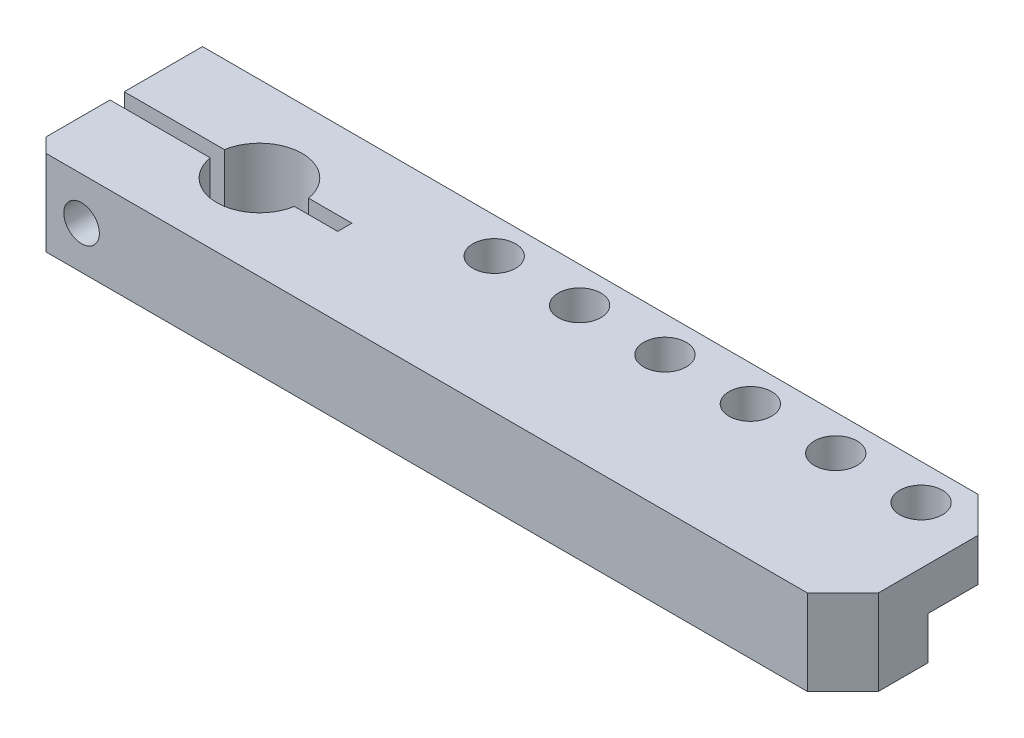
from build123d import *

# Parameters (mm, degrees)
SKETCH1_W                = 65
SKETCH1_H                = 12
SKETCH1_R                = 3
BOSS_EXTRUDE1_DEPTH      = 6
SKETCH2_W                = 32
SKETCH2_H                = 1
CUT_EXTRUDE1_DEPTH       = 34.589432862
SKETCH4_R                = 1.75
CUT_EXTRUDE3_DEPTH       = 6
M3_TAPPED_HOLE1_D        = 2.5
SKETCH10_W               = 48
SKETCH10_H               = 6
CUT_EXTRUDE4_DEPTH       = 3
F_3_0_3_DIAMETER_HOLE1_D = 3
LPATTERN1_COUNT          = 6
LPATTERN1_PITCH          = 6
FILLET1_R                = 3
SKETCH11_W               = 8
SKETCH11_H               = 12
CUT_EXTRUDE5_DEPTH       = 10
CHAMFER1_SIZE            = 1
CHAMFER2_SIZE            = 2.5


with BuildPart() as part:
    # Sketch1 → Boss-Extrude1 (new body)
    with BuildSketch(Plane(origin=(0, 0, 0), x_dir=(1, 0, 0), z_dir=(0, 1, 0))):
        Rectangle(SKETCH1_W, SKETCH1_H)
        with Locations(Location((-22.5, 0, 0), (0, 0, 270))):
            Circle(SKETCH1_R, mode=Mode.SUBTRACT)
    extrude(amount=BOSS_EXTRUDE1_DEPTH)

    # Sketch2 → Cut-Extrude1 (cut, through all)
    with BuildSketch(Plane.XZ):
        with Locations((-32.5, 0)):
            Rectangle(SKETCH2_W, SKETCH2_H)
    extrude(amount=-CUT_EXTRUDE1_DEPTH, mode=Mode.SUBTRACT)

    # Sketch4 → Cut-Extrude3 (cut)
    with BuildSketch(Plane(origin=(0, 0, -6), x_dir=(-1, 0, 0), z_dir=(0, 0, -1))):
        with Locations((29, 3)):
            Circle(SKETCH4_R)
    extrude(amount=-CUT_EXTRUDE3_DEPTH, mode=Mode.SUBTRACT)

    # M3 Tapped Hole1 (through all)
    with Locations(Plane(origin=(-29, 3, 0.5), x_dir=(-1, 0, 0), z_dir=(0, 0, -1))):
        with Locations((0, 0)):
            Hole(M3_TAPPED_HOLE1_D / 2)

    # Sketch10 → Cut-Extrude4 (cut)
    with BuildSketch(Plane.XZ):
        with Locations((8.5, -3)):
            Rectangle(SKETCH10_W, SKETCH10_H)
    extrude(amount=-CUT_EXTRUDE4_DEPTH, mode=Mode.SUBTRACT)

    # Ø3.0 (3) Diameter Hole1 (through all)
    with Locations(Plane(origin=(20.5, 0, -3.5), x_dir=(0, 0, -1), z_dir=(0, -1, 0))):
        with Locations((0, 0)):
            f_3_0_3_diameter_hole1 = Hole(F_3_0_3_DIAMETER_HOLE1_D / 2)

    # LPattern1: Ø3.0 (3) Diameter Hole1 ×6
    with Locations(*[(-i * LPATTERN1_PITCH, 0, 0) for i in range(1, LPATTERN1_COUNT)]):
        add(f_3_0_3_diameter_hole1, mode=Mode.SUBTRACT)

    # Fillet1
    fillet1_edges = [part.edges().sort_by_distance(p)[0] for p in [
        (-15.5, 1.5, 0),
    ]]
    fillet(fillet1_edges, radius=FILLET1_R)

    # Sketch11 → Cut-Extrude5 (cut)
    with BuildSketch(Plane.XZ):
        with Locations((28.5, 0)):
            Rectangle(SKETCH11_W, SKETCH11_H)
    extrude(amount=-CUT_EXTRUDE5_DEPTH, mode=Mode.SUBTRACT)

    # Chamfer1
    chamfer1_edges = [part.edges().sort_by_distance(p)[0] for p in [
        (-32.5, 3, 6),
    ]]
    chamfer(chamfer1_edges, length=CHAMFER1_SIZE)

    # Chamfer2
    chamfer2_edges = [part.edges().sort_by_distance(p)[0] for p in [
        (24.5, 4.5, -6),
        (24.5, 3, 6),
    ]]
    chamfer(chamfer2_edges, length=CHAMFER2_SIZE)


solid = part.part
